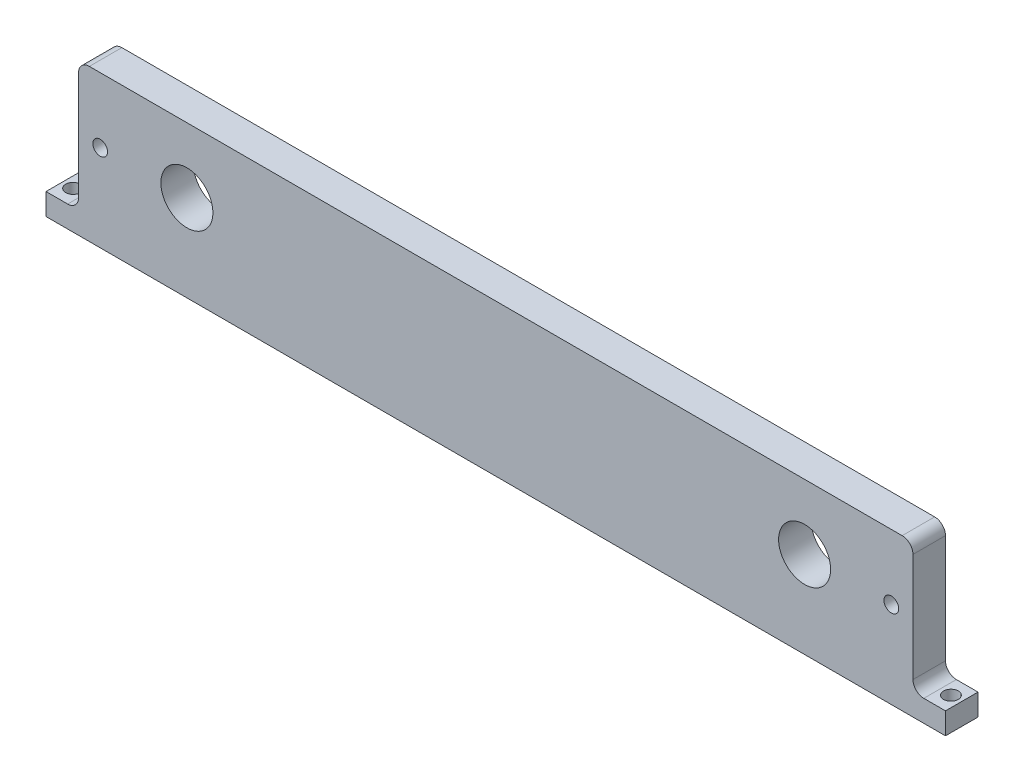
SolidWorks part; units mm, degrees
material "6061合金"
ref_plane "Front Plane" through (0, 0, 0) normal (0, 0, 1) x (1, 0, 0)
ref_plane "Top Plane" through (0, 0, 0) normal (0, 1, 0) x (1, 0, 0)
ref_plane "Right Plane" through (0, 0, 0) normal (1, 0, 0) x (0, 0, -1)
sketch "Sketch1" plane through (0, 0, 0) normal (0, 0, 1) x (1, 0, 0)
  line L1 (207.5, -35) -> (-207.5, -35)
  line L2 (207.5, -35) -> (207.5, 35)
  line L3 (207.5, 35) -> (-207.5, 35)
  line L4 (-207.5, -35) -> (-207.5, 35)
  line L5 (207.5, -35) -> (-207.5, 35) construction
  line L6 (207.5, 35) -> (-207.5, -35) construction
  point P0 (0, 0)
  dimension "D1" = 415
  dimension "D2" = 70
extrude "Boss-Extrude1" add sketch "Sketch1" along normal blind 15
sketch "Sketch2" plane through (0, 0, 15) normal (0, 0, 1) x (1, 0, 0)
  line L0 (-182.5, 5) -> (-142.5, 5) construction
  line L1 (-142.5, 5) -> (142.5, 5) construction
  line L2 (142.5, 5) -> (182.5, 5) construction
  line L3 (0, 35) -> (0, 5) construction
  line L6 (-207.5, 35) -> (-207.5, -35) construction
  line L7 (207.5, 35) -> (-207.5, 35) construction
  line L8 (-207.5, -35) -> (207.5, -35) construction
  circle A0 centre (-182.5, 5) radius 3.4
  circle A1 centre (-142.5, 5) radius 12
  circle A3 centre (142.5, 5) radius 12
  circle A4 centre (182.5, 5) radius 3.4
  dimension "D1" = 6.8
  dimension "D2" = 24
  dimension "D3" = 40
  dimension "D6" = 365
  dimension "D7" = 40
  dimension "D5" = 40
  dimension "D11" = 25
extrude "Cut-Extrude1" cut sketch "Sketch2" against normal through all
sketch "Sketch10" plane through (0, 0, 15) normal (0, 0, 1) x (1, 0, 0)
  line L0 (0, 0) -> (0, 35) construction
  line L1 (-207.5, 35) -> (-192.5, 35)
  line L2 (-207.5, 35) -> (-207.5, -25)
  line L3 (-207.5, -25) -> (-192.5, -25)
  line L4 (-192.5, 35) -> (-192.5, -25)
  line L5 (207.5, 35) -> (-207.5, 35) construction
  line L6 (192.5, 35) -> (192.5, -25)
  line L7 (207.5, -25) -> (192.5, -25)
  line L8 (207.5, 35) -> (207.5, -25)
  line L9 (207.5, 35) -> (192.5, 35)
  line L10 (-207.5, -35) -> (207.5, -35) construction
  dimension "D1" = 15
  dimension "D2" = 10
extrude "Cut-Extrude2" cut sketch "Sketch10" against normal through all
hole_wizard "Ø6.8 (6.8) Diameter Hole1" positions "Sketch11" profile "Sketch12" hole size "Ø6.8" standard "GB"
sketch "Sketch11" plane through (0, -35, 0) normal (0, -1, 0) x (-1, 0, 0)
  line L0 (-207.5, -7.5) -> (-202.5, -7.5) construction
  line L1 (-207.5, -15) -> (-207.5, 0) construction
  line L3 (207.5, -7.5) -> (202.5, -7.5) construction
  line L4 (207.5, -15) -> (207.5, 0) construction
  point P0 (-202.5, -7.5)
  point P9 (202.5, -7.5)
  dimension "D1" = 5
  dimension "D2" = 5
sketch "Sketch12" plane through (202.5, -35, 7.5) normal (1, 0, 0) x (0, 0, -1)
  line L0 (0, 0) -> (0, 14.4429)
  line L1 (0, 14.4429) -> (3.4, 12.4)
  line L2 (3.4, 12.4) -> (3.4, 0)
  line L5 (3.4, 0) -> (0, 0)
  line L10 (0, 14.4429) -> (-3.4, 12.4) construction
  line L11 (0, -6.35) -> (0, 107.95) construction
  dimension "孔直径" = 6.8
  dimension "孔深度" = 12.4
  dimension "导头角度" = 118
fillet "Fillet1" radius 5 2 edges at (192.5, -25, 7.5) (-192.5, -25, 7.5)
fillet "Fillet2" radius 5 2 edges at (-192.5, 35, 7.5) (192.5, 35, 7.5)
hole_wizard "M6 Tapped Hole1" positions "Sketch13" profile "Sketch14" tap size "M6" standard "GB"
sketch "Sketch13" plane through (0, -35, 0) normal (0, -1, 0) x (-1, 0, 0)
  line L0 (125, -7.5) -> (-125, -7.5) construction
  line L2 (0, 0) -> (0, -7.5) construction
  line L4 (207.5, -7.5) -> (125, -7.5) construction
  line L5 (207.5, -15) -> (207.5, 0) construction
  point P0 (125, -7.5)
  point P2 (-125, -7.5)
  dimension "D1" = 250
sketch "Sketch14" plane through (-125, -35, 7.5) normal (1, 0, 0) x (0, 0, -1)
  line L0 (0, 0) -> (0, 16.5022)
  line L1 (0, 16.5022) -> (2.5, 15)
  line L2 (2.5, 15) -> (2.5, 0)
  line L5 (2.5, 0) -> (0, 0)
  line L10 (0, 16.5022) -> (-2.5, 15) construction
  line L11 (0, -6.35) -> (0, 107.95) construction
  dimension "螺纹孔钻头直径" = 5
  dimension "螺纹孔钻头深度" = 15
  dimension "导头角度" = 118
cosmetic thread "Hole Thread1" parameters "D1"=12, "D2"=6
cosmetic thread "Hole Thread2" parameters "D1"=12, "D2"=6
